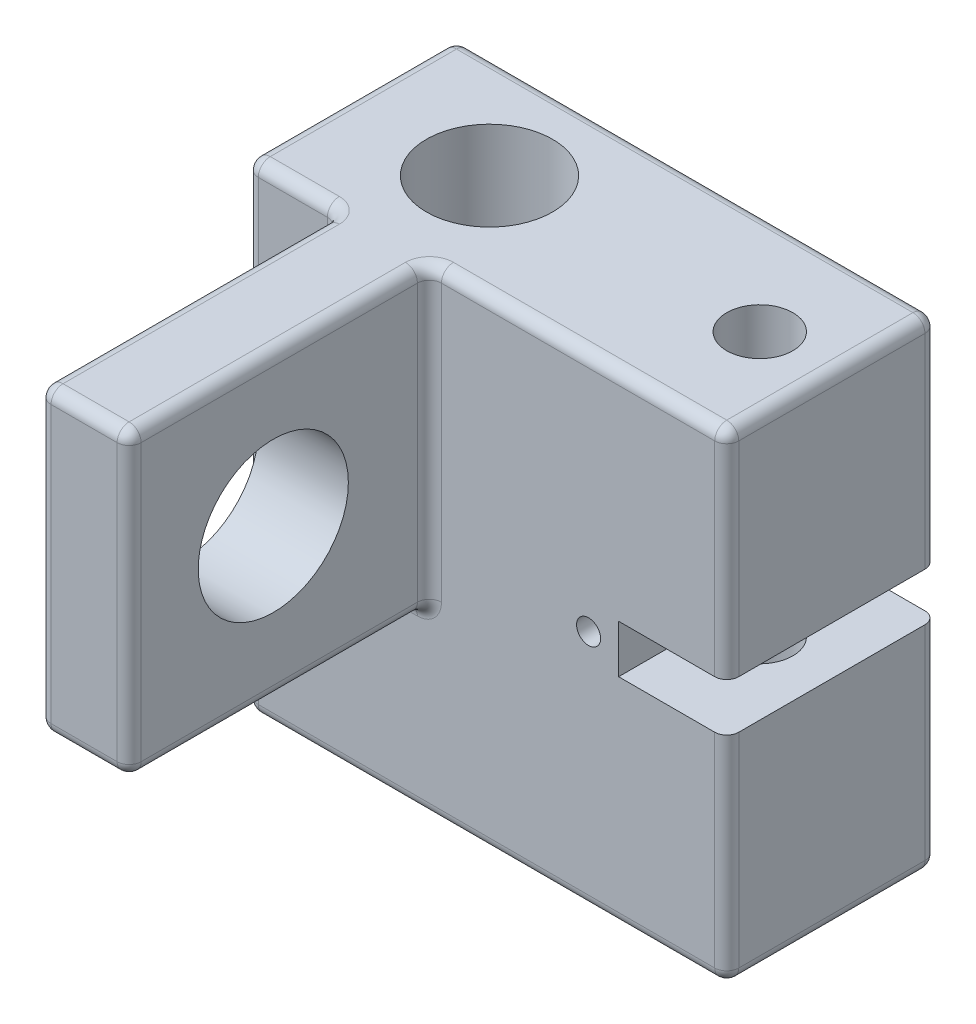
from build123d import *

# Parameters (mm, degrees)
SKETCH1_W           = 80
SKETCH1_H           = 35
SKETCH1_R           = 5.5
SKETCH1_R_2         = 10.5
SKETCH1_W_2         = 15
SKETCH1_H_2         = 50
BOSS_EXTRUDE1_DEPTH = 40
SKETCH2_R           = 6
CUT_EXTRUDE1_DEPTH  = 10
SKETCH4_W           = 50
SKETCH4_H           = 30
CUT_EXTRUDE3_DEPTH  = 81.933614772
SKETCH3_R           = 12.5
CUT_EXTRUDE2_DEPTH  = 15
SKETCH6_W           = 18
SKETCH6_H           = 8
CUT_EXTRUDE4_DEPTH  = 103.46950766
FILLET1_R           = 2
SKETCH7_R           = 2
CUT_EXTRUDE5_DEPTH  = 103.46950766


with BuildPart() as part:
    # Sketch1 → Boss-Extrude1 (new, symmetric)
    # profile 1 of 2: a face of its own
    with BuildSketch(Plane(origin=(0, 0, 0), x_dir=(1, 0, 0), z_dir=(0, 1, 0))):
        with Locations((40, 17.5)):
            Rectangle(SKETCH1_W, SKETCH1_H)
        with Locations(Location((68, 17.5, 0), (0, 0, 270))):
            Circle(SKETCH1_R, mode=Mode.SUBTRACT)
        with Locations(Location((23, 17.5, 0), (0, 0, 270))):
            Circle(SKETCH1_R_2, mode=Mode.SUBTRACT)
    # profile 2 of 2: a face of its own
    with BuildSketch(Plane(origin=(0, 0, 0), x_dir=(1, 0, 0), z_dir=(0, 1, 0))):
        with Locations((23, -25)):
            Rectangle(SKETCH1_W_2, SKETCH1_H_2)
    extrude(amount=BOSS_EXTRUDE1_DEPTH, both=True)

    # Sketch2 → Cut-Extrude1 (cut)
    with BuildSketch(Plane.ZY):
        with Locations((-17.5, 22.5)):
            Circle(SKETCH2_R)
        with Locations((-17.5, -22.5)):
            Circle(SKETCH2_R)
    extrude(amount=-CUT_EXTRUDE1_DEPTH, mode=Mode.SUBTRACT)

    # Sketch4 → Cut-Extrude3 (cut, through all)
    with BuildSketch(Plane(origin=(30.5, 0, 0), x_dir=(0, 0, -1), z_dir=(1, 0, 0))):
        with Locations((-25, -25)):
            Rectangle(SKETCH4_W, SKETCH4_H)
    extrude(amount=-CUT_EXTRUDE3_DEPTH, mode=Mode.SUBTRACT)

    # Sketch3 → Cut-Extrude2 (cut)
    with BuildSketch(Plane(origin=(30.5, 0, 0), x_dir=(0, 0, -1), z_dir=(1, 0, 0))):
        with Locations((-26, 15)):
            Circle(SKETCH3_R)
    extrude(amount=-CUT_EXTRUDE2_DEPTH, mode=Mode.SUBTRACT)

    # Sketch6 → Cut-Extrude4 (cut, through all)
    with BuildSketch(Plane.XY):
        with Locations((71, 0)):
            Rectangle(SKETCH6_W, SKETCH6_H)
    extrude(amount=-CUT_EXTRUDE4_DEPTH, mode=Mode.SUBTRACT)

    # Fillet1
    fillet1_edges = [part.edges().sort_by_distance(p)[0] for p in [
        (55.25, 40, 0),
        (40, -40, 0),
        (0, -40, -17.5),
        (40, -40, -35),
        (80, 40, -17.5),
        (80, -40, -17.5),
        (40, 40, -35),
        (30.5, 15, 50),
        (15.5, 15, 50),
        (15.5, 15, 0),
        (0, 0, 0),
        (0, 0, -35),
        (80, 22, -35),
        (80, 22, 0),
        (30.5, 15, 0),
        (0, 40, -17.5),
        (7.75, 40, 0),
        (15.5, 40, 25),
        (23, 40, 50),
        (15.5, -10, 25),
        (23, -10, 50),
        (23, -10, 0),
        (30.5, -10, 25),
        (30.5, 40, 25),
        (80, -22, 0),
        (80, -22, -35),
    ]]
    fillet(fillet1_edges, radius=FILLET1_R)

    # Sketch7 → Cut-Extrude5 (cut, through all)
    with BuildSketch(Plane.XY):
        with Locations((57, 0)):
            Circle(SKETCH7_R)
    extrude(amount=-CUT_EXTRUDE5_DEPTH, mode=Mode.SUBTRACT)


solid = part.part
